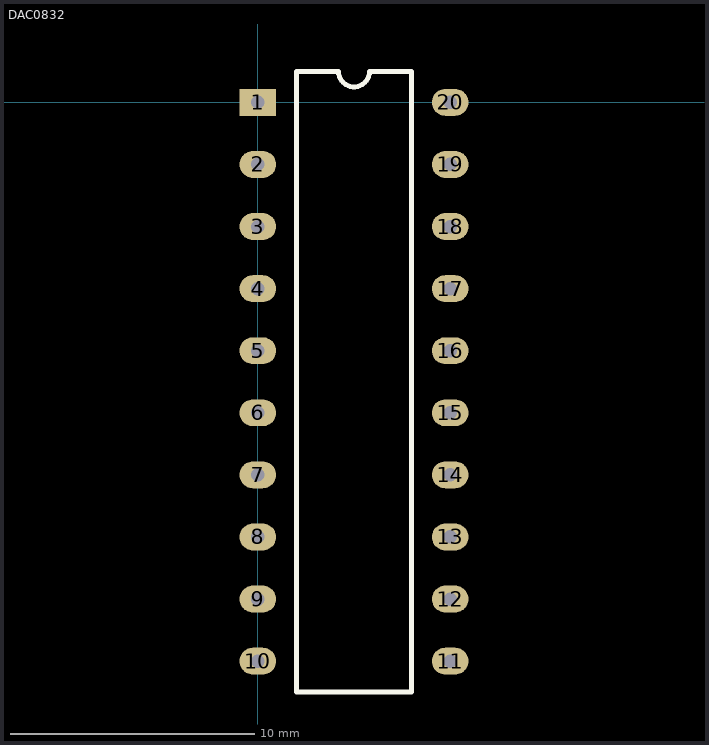
[diagram p0: the footprints below, top view; thin cyan lines are the x and y axes]
# Altium footprint library MISC89340-6.PcbLib: 2 footprints
Each footprint in its own frame and in the unit in brackets; x right, y up, seen from the top. Pads: shape width x height; smd on the part's side, far side on the other; paste and mask are expansions set on the pad; w line width, h text height; cw(c..) or ccw(c..) is an arc to the next point about the centre after c.

## DAC0832 [mm]
pads (20):
  rect 1.5x1.1 hole 0.55: 1(0,0)
  oval 1.5x1.1 hole 0.55: 2(0,-2.54) 3(0,-5.08) 4(0,-7.62) 5(0,-10.16) 6(0,-12.7) 7(0,-15.24) 8(0,-17.78) 9(0,-20.32) 10(0,-22.86) 11(7.87,-22.86) 12(7.87,-20.32) 13(7.87,-17.78) 14(7.87,-15.24) 15(7.87,-12.7) 16(7.87,-10.16) 17(7.87,-7.62) 18(7.87,-5.08) 19(7.87,-2.54) 20(7.87,0)
Top Overlay:
  lines w0.2: 1.585,-24.13 1.585,1.27 3.3,1.27 ccw(c3.935,1.27) 4.57,1.27 6.285,1.27 6.285,-24.13 1.585,-24.13

## PCBComponent_1 [mm]